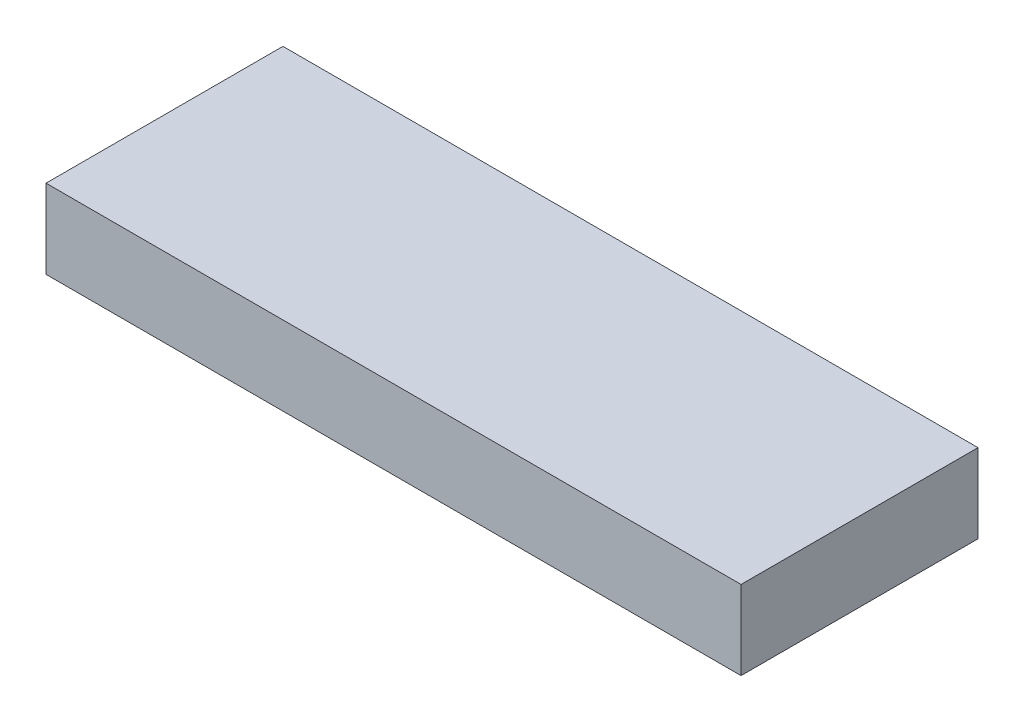
from build123d import *

# Parameters (mm, degrees)
SKETCH_1_W      = 44
SKETCH_1_H      = 15
EXTRUDE_1_DEPTH = 5


with BuildPart() as part:
    # 草图1 → 凸台-拉伸1 (new body)
    with BuildSketch(Plane(origin=(0, 0, 0), x_dir=(1, 0, 0), z_dir=(0, 1, 0))):
        Rectangle(SKETCH_1_W, SKETCH_1_H)
    extrude(amount=EXTRUDE_1_DEPTH)


solid = part.part
